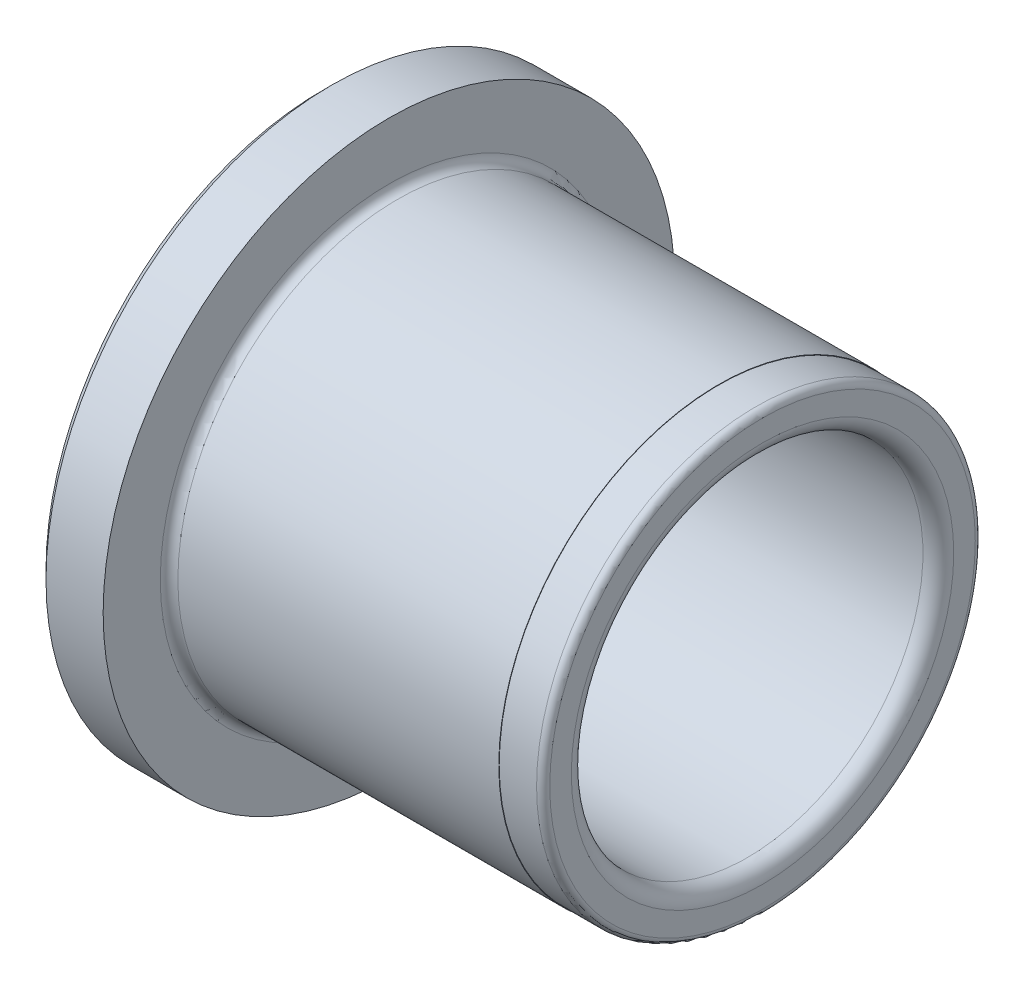
SolidWorks part; units mm, degrees
material "H62"
ref_plane "Front Plane" through (0, 0, 0) normal (0, 0, 1) x (1, 0, 0)
ref_plane "Top Plane" through (0, 0, 0) normal (0, 1, 0) x (1, 0, 0)
ref_plane "Right Plane" through (0, 0, 0) normal (1, 0, 0) x (0, 0, -1)
sketch "Sketch1" plane through (0, 0, 0) normal (0, 0, 1) x (1, 0, 0)
  line L0 (0, 12.6) -> (0, 9.1164)
  line L1 (0.5784, 8.427) -> (3, 8)
  line L2 (3, 8) -> (19.3, 8)
  line L3 (20, 8.7) -> (20, 9.68)
  line L4 (19.7, 9.98) -> (18, 9.98)
  line L5 (18, 9.98) -> (18, 10)
  line L6 (18, 10) -> (3.4, 10)
  line L7 (3, 10.4) -> (3, 13)
  line L8 (3, 13) -> (0.4, 13)
  line L9 (0.4, 13) -> (0, 12.6)
  line L10 (20, 0) -> (0, 0) construction
  arc A0 (0, 9.1164) -> (0.5784, 8.427) centre (0.7, 9.1164) ccw
  arc A1 (19.3, 8) -> (20, 8.7) centre (19.3, 8.7) ccw
  arc A2 (20, 9.68) -> (19.7, 9.98) centre (19.7, 9.68) ccw
  arc A3 (3.4, 10) -> (3, 10.4) centre (3.4, 10.4) cw
revolve "Revolve1" add sketch "Sketch1" angle 360 about L10
